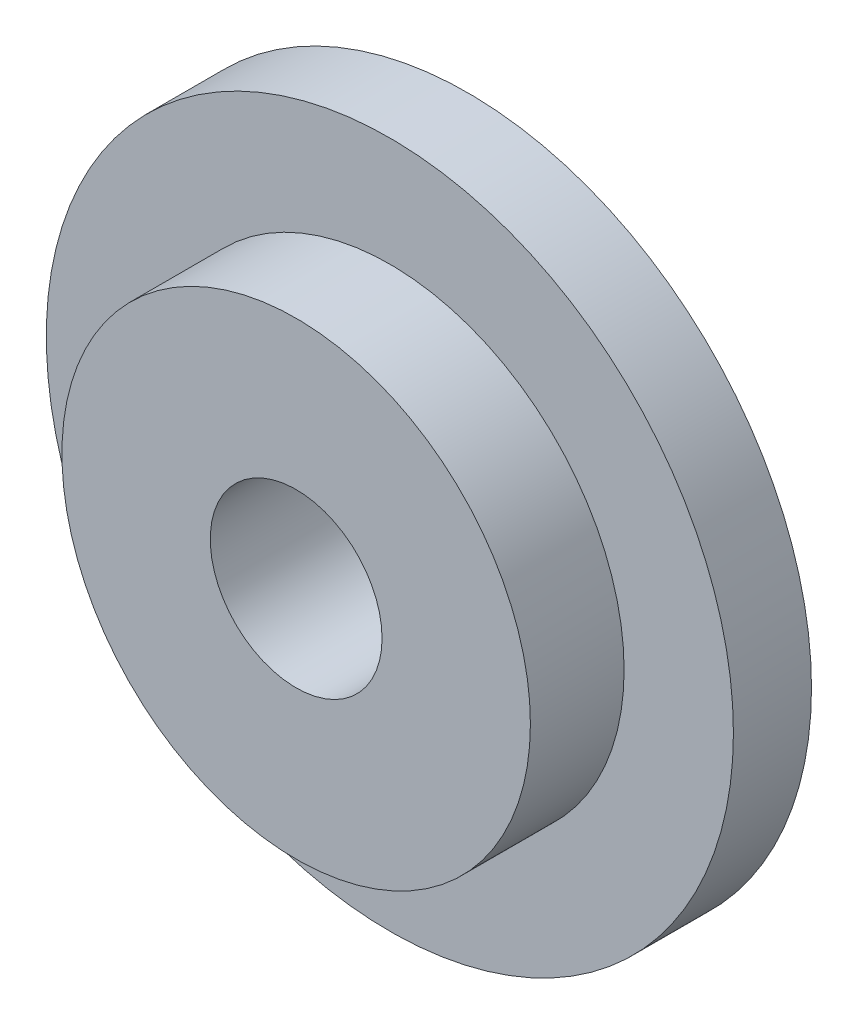
from build123d import *


with BuildPart() as part:
    # Sketch1 → Revolve1 (revolve)
    with BuildSketch(Plane(origin=(0, 0, 0), x_dir=(0, 0, -1), z_dir=(1, 0, 0)), mode=Mode.PRIVATE) as revolve1_sk:
        Polygon((0, 15), (0, 5.5), (9, 5.5), (11, 8.964101615), (11, 22), (6, 22), (6, 15), align=None)
    revolve(revolve1_sk.sketch.rotate(Axis((0, 0, 17.908444602), (0, 0, -1)), 90), axis=Axis((0, 0, 17.908444602), (0, 0, -1)))


solid = part.part
